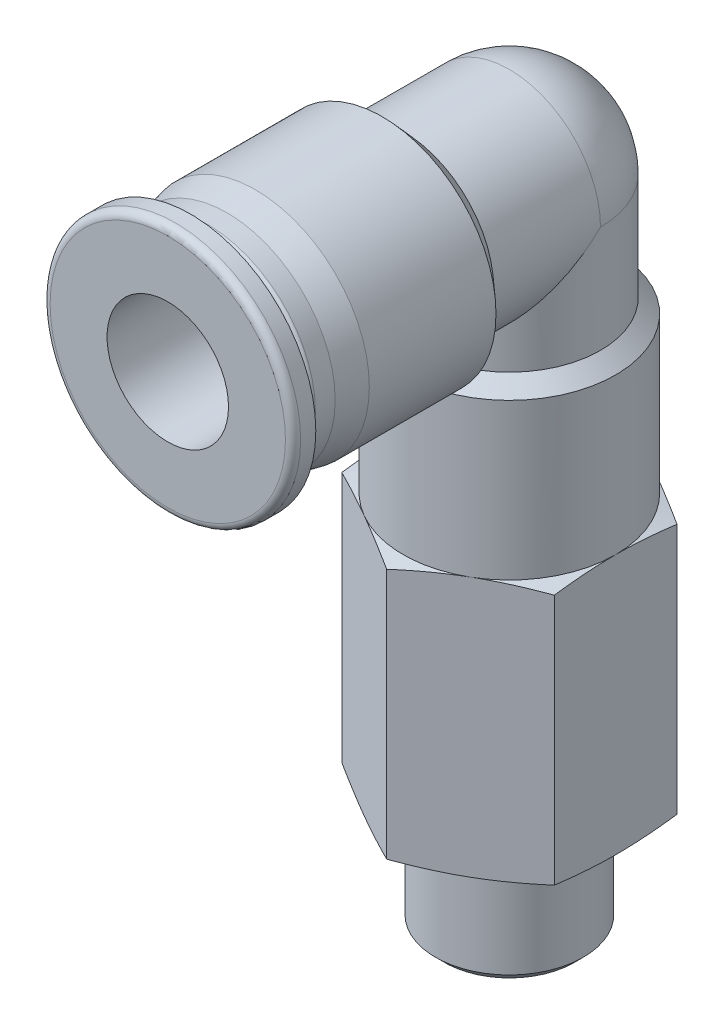
SolidWorks part; units mm, degrees
ref_plane "前视基准面" through (0, 0, 0) normal (0, 0, 1) x (1, 0, 0)
ref_plane "上视基准面" through (0, 0, 0) normal (0, 1, 0) x (1, 0, 0)
ref_plane "右视基准面" through (0, 0, 0) normal (1, 0, 0) x (0, 0, -1)
sketch "草图1" plane through (0, 0, 0) normal (1, 0, 0) x (0, 0, -1)
  line L0 (-22.5, 0) -> (-22.5, 7.75)
  line L1 (-22, 8.25) -> (-21, 8.25)
  line L2 (-21, 8.25) -> (-21, 6)
  line L3 (-21, 6) -> (-20.1, 6)
  line L4 (-20.1, 6) -> (-20.1, 6.925)
  line L5 (-19.9, 7.125) -> (-18.6, 7.125)
  line L6 (-18.6, 7.125) -> (-16.725, 7.5)
  line L7 (-16.725, 7.5) -> (-8.3819, 7.5)
  line L8 (-8.3819, 7.5) -> (-7.0312, 6)
  line L9 (-7.0312, 6) -> (0, 6)
  line L10 (6, 0) -> (-22.5, 0)
  line L11 (6, 0) -> (-22.5, 0) construction
  arc A0 (-22.5, 7.75) -> (-22, 8.25) centre (-22, 7.75) cw
  arc A1 (-20.1, 6.925) -> (-19.9, 7.125) centre (-19.9, 6.925) cw
  arc A2 (0, 6) -> (6, 0) centre (0, 0) cw
revolve "旋转1" add sketch "草图1" angle 360 about L11
sketch "草图2" plane through (0, 0, 0) normal (1, 0, 0) x (0, 0, -1)
  line L0 (0, -42.8) -> (-4.283, -42.8)
  line L1 (-4.283, -42.8) -> (-4.864, -42.219)
  line L2 (-4.864, -42.219) -> (-4.864, -35.8723)
  line L3 (-4.864, -35.8723) -> (-8.0829, -35.0098)
  line L4 (-8.0829, -35.0098) -> (-8.0829, -18.4702)
  line L5 (-8.0829, -18.4702) -> (-7, -18.18)
  line L6 (-7, -18.18) -> (-7, -7.9317)
  line L7 (-7, -7.9317) -> (-6, -7.0312)
  line L8 (-6, -7.0312) -> (-6, 0)
  line L9 (-6, 0) -> (0, 0)
  line L10 (0, 0) -> (0, -42.8)
  line L11 (0, 0) -> (0, -42.8) construction
revolve "旋转2" add sketch "草图2" angle 360 about L11
cosmetic thread "装饰螺纹线1" parameters "D1"=6.9277, "D2"=8.566
ref_plane "基准面4" through (0, -35.3, 0) normal (0, 1, 0) x (1, 0, 0)
sketch "草图3" plane through (0, -35.3, 0) normal (0, 1, 0) x (1, 0, 0)
  line L0 (-7, 4.0415) -> (-7, -4.0415)
  line L1 (-7, -4.0415) -> (0, -8.0829)
  line L2 (0, -8.0829) -> (7, -4.0415)
  line L3 (7, -4.0415) -> (7, 4.0415)
  line L4 (7, 4.0415) -> (0, 8.0829)
  line L5 (0, 8.0829) -> (-7, 4.0415)
  circle A0 centre (0, 0) radius 14
extrude "切除-拉伸1" cut sketch "草图3" along normal blind 21.4
sketch "草图4" plane through (0, 0, 0) normal (1, 0, 0) x (0, 0, -1)
  line L0 (-22.5, 0) -> (-22.5, 4)
  line L1 (-22.5, 4) -> (0, 4)
  line L2 (4, 0) -> (-22.5, 0)
  line L3 (4, 0) -> (-22.5, 0) construction
  arc A0 (0, 4) -> (4, 0) centre (0, 0) cw
revolve "切除-旋转1" cut sketch "草图4" angle 360 about L3
sketch "草图5" plane through (0, 0, 0) normal (1, 0, 0) x (0, 0, -1)
  line L0 (0, -42.8) -> (-2.6667, -42.8)
  line L1 (-2.6667, -42.8) -> (-2.6667, 0)
  line L2 (-2.6667, 0) -> (0, 0)
  line L3 (0, 0) -> (0, -42.8)
  line L4 (0, 0) -> (0, -42.8) construction
revolve "切除-旋转2" cut sketch "草图5" angle 360 about L4
